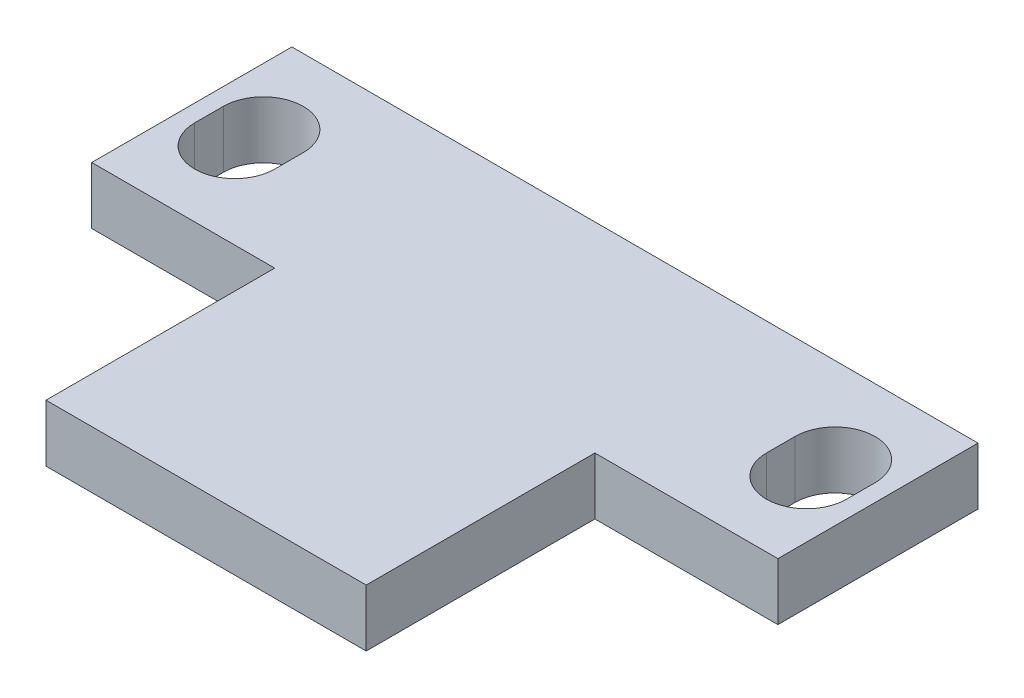
from build123d import *

# Parameters (mm, degrees)
BOSS_EXTRUDE1_DEPTH = 10


with BuildPart() as part:
    # Sketch1 → Boss-Extrude1 (new body)
    with BuildSketch(Plane(origin=(0, 0, 0), x_dir=(1, 0, 0), z_dir=(0, 1, 0))):
        Polygon((-60, 37.5), (-60, 2.5), (-28, 2.5), (-28, -37.5), (28, -37.5), (28, 2.5), (60, 2.5), (60, 37.5), align=None)
        with BuildLine():
            ThreePointArc((-57, 22.5), (-50, 29.5), (-43, 22.5))
            Line((-43, 22.5), (-43, 17.5))
            ThreePointArc((-43, 17.5), (-50, 10.5), (-57, 17.5))
            Line((-57, 17.5), (-57, 22.5))
        make_face(mode=Mode.SUBTRACT)
        with BuildLine():
            Line((43, 17.5), (43, 22.5))
            ThreePointArc((43, 22.5), (50, 29.5), (57, 22.5))
            Line((57, 22.5), (57, 17.5))
            ThreePointArc((57, 17.5), (50, 10.5), (43, 17.5))
        make_face(mode=Mode.SUBTRACT)
    extrude(amount=BOSS_EXTRUDE1_DEPTH)


solid = part.part
